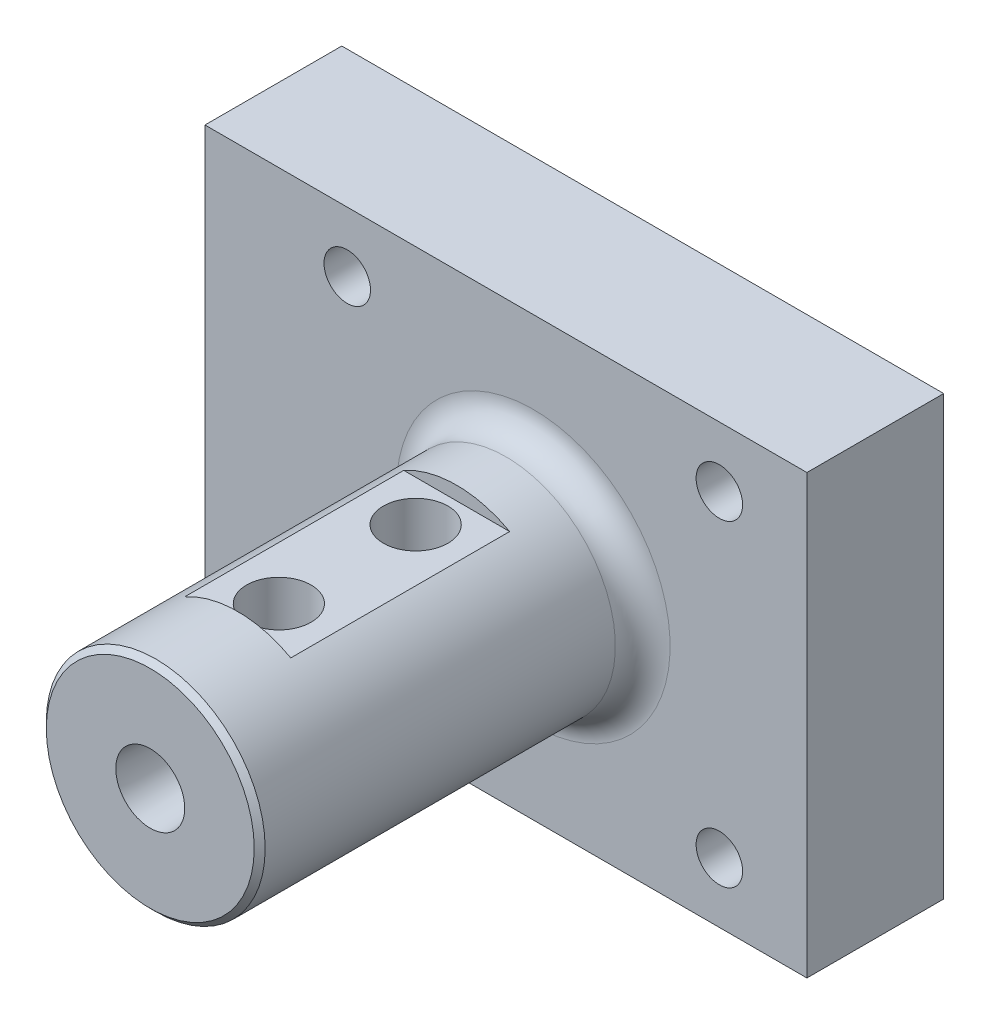
SolidWorks part; units mm, degrees
material "T2"
ref_plane "前视基准面" through (0, 0, 0) normal (0, 0, 1) x (1, 0, 0)
ref_plane "上视基准面" through (0, 0, 0) normal (0, 1, 0) x (1, 0, 0)
ref_plane "右视基准面" through (0, 0, 0) normal (1, 0, 0) x (0, 0, -1)
sketch "草图13" plane through (0, 0, 0) normal (0, 0, 1) x (1, 0, 0)
  line L1 (-50, -40) -> (50, -40)
  line L2 (-50, -40) -> (-50, 40)
  line L3 (-50, 40) -> (50, 40)
  line L4 (50, -40) -> (50, 40)
  line L5 (0, 40) -> (0, -40) construction
  line L6 (-50, 0) -> (50, 0) construction
  point P0 (0, 0)
  dimension "D1" = 100
  dimension "D2" = 80
extrude "凸台-拉伸3" add sketch "草图13" along normal blind 25
sketch "草图14" plane through (0, 0, 25) normal (0, 0, 1) x (1, 0, 0)
  line L1 (-34, -29) -> (34, -29) construction
  line L2 (-34, -29) -> (-34, 29) construction
  line L3 (-34, 29) -> (34, 29) construction
  line L4 (34, -29) -> (34, 29) construction
  line L5 (0, 29) -> (0, -29) construction
  line L6 (-34, 0) -> (34, 0) construction
  circle A0 centre (-34, 29) radius 0.5
  circle A1 centre (34, 29) radius 0.5
  circle A2 centre (34, -29) radius 0.5
  circle A3 centre (-34, -29) radius 0.5
  point P0 (0, 0)
  dimension "D3" = 1
  dimension "D1" = 68
  dimension "D2" = 58
extrude "切除-拉伸4" cut sketch "草图14" against normal blind 18
sketch "草图15" plane through (0, 0, 25) normal (0, 0, 1) x (1, 0, 0)
  circle A0 centre (0, 0) radius 20
  dimension "D1" = 40
extrude "凸台-拉伸4" add sketch "草图15" along normal blind 70
hole_wizard "Ø10.0 (10) 直径孔1" positions "草图16" profile "草图17" hole size "Ø10.0" standard "GB"
sketch "草图16" plane through (0, 0, 95) normal (0, 0, 1) x (1, 0, 0)
  point P5 (0, 0)
sketch "草图17" plane through (0, 0, 95) normal (1, 0, 0) x (0, -1, 0)
  line L0 (0, 0) -> (0, 28.0043)
  line L1 (0, 28.0043) -> (5, 25)
  line L2 (5, 25) -> (5, 0)
  line L5 (5, 0) -> (0, 0)
  line L10 (0, 28.0043) -> (-5, 25) construction
  line L11 (0, -6.35) -> (0, 107.95) construction
  dimension "孔直径" = 10
  dimension "孔深度" = 25
  dimension "导头角度" = 118
sketch "草图19" plane through (0, 0, 0) normal (0, 1, 0) x (1, 0, 0)
  line L0 (0, -95) -> (0, 0) construction
  line L1 (-20, -95) -> (20, -95) construction
  line L2 (0, -95) -> (-0.5, -95) construction
  line L3 (-0.5, -95) -> (0, -85) construction
  line L4 (0, -95) -> (-0.5, -95)
  line L5 (-6.3, -95) -> (-5.65, -82)
  line L6 (-5.65, -82) -> (-5, -82)
  line L8 (-5, -82) -> (-5, -95)
  line L10 (0, -95) -> (-0.5, -95)
  line L11 (-5, -70) -> (-5, -95) construction
  line L12 (-5, -95) -> (-6.3, -95)
  dimension "D1" = 0.5
  dimension "D2" = 10
  dimension "D3" = 12.6
  dimension "D4" = 13
revolve "切除-旋转10" cut sketch "草图19" angle 360 about L0
ref_plane "基准面3" through (0, 0, 79) normal (0, 0, 1) x (1, 0, 0)
sketch "草图21" plane through (0, 0, 79) normal (0, 0, 1) x (1, 0, 0)
  line L1 (-27.2886, -17.5) -> (27.2886, -17.5)
  line L2 (-27.2886, -17.5) -> (-27.2886, 17.5)
  line L3 (-27.2886, 17.5) -> (27.2886, 17.5)
  line L4 (27.2886, -17.5) -> (27.2886, 17.5)
  line L5 (0, 17.5) -> (0, -17.5) construction
  line L6 (-27.2886, 0) -> (27.2886, 0) construction
  point P0 (0, 0)
  dimension "D1" = 35
extrude "切除-拉伸5" cut sketch "草图21" against normal blind 40 flip side to cut
hole_wizard "G1/4 螺纹孔1" positions "草图22" profile "草图23" tap size "G1/4" standard "GB"
sketch "草图22" plane through (0, 17.5, 0) normal (0, 1, 0) x (1, 0, 0)
  line L0 (0, 0) -> (0, -95) construction
  line L1 (-20, -95) -> (20, -95) construction
  line L2 (-9.6825, -59) -> (9.6825, -59) construction
  line L3 (-9.6825, -39) -> (-9.6825, -79) construction
  line L4 (9.6825, -79) -> (9.6825, -39) construction
  point P13 (0, -46.5)
  point P15 (0, -71.5)
  dimension "D1" = 25
sketch "草图23" plane through (0, 17.5, 71.5) normal (1, 0, 0) x (0, 0, 1)
  line L0 (0, 0) -> (0, 28.5451)
  line L1 (0, 28.5451) -> (5.9, 25)
  line L2 (5.9, 25) -> (5.9, 0)
  line L5 (5.9, 0) -> (0, 0)
  line L10 (0, 28.5451) -> (-5.9, 25) construction
  line L11 (0, -6.35) -> (0, 107.95) construction
  dimension "螺纹孔钻头直径" = 11.8
  dimension "螺纹孔钻头深度" = 25
  dimension "导头角度" = 118
cosmetic thread "孔螺蚊线5" parameters "D1"=20, "D2"=13.157
cosmetic thread "孔螺蚊线6" parameters "D1"=20, "D2"=13.157
chamfer "倒角1" distance 1 angle 45 1 edges at (20, 0, 95)
hole_wizard "M10 螺纹孔1" positions "草图24" profile "草图25" tap size "M10" standard "GB"
sketch "草图24" plane through (0, 0, 25) normal (0, 0, 1) x (1, 0, 0)
  point P4 (-34, 29)
  point P7 (34, 29)
  point P10 (34, -29)
  point P13 (-34, -29)
sketch "草图25" plane through (-34, 29, 25) normal (1, 0, 0) x (0, -1, 0)
  line L0 (0, 0) -> (0, 30.0537)
  line L1 (0, 30.0537) -> (4.25, 27.5)
  line L2 (4.25, 27.5) -> (4.25, 0)
  line L5 (4.25, 0) -> (0, 0)
  line L10 (0, 30.0537) -> (-4.25, 27.5) construction
  line L11 (0, -6.35) -> (0, 107.95) construction
  dimension "螺纹孔钻头直径" = 8.5
  dimension "螺纹孔钻头深度" = 27.5
  dimension "导头角度" = 118
cosmetic thread "孔螺蚊线7" parameters "D1"=18, "D2"=10
cosmetic thread "孔螺蚊线8" parameters "D1"=18, "D2"=10
cosmetic thread "孔螺蚊线9" parameters "D1"=18, "D2"=10
cosmetic thread "孔螺蚊线10" parameters "D1"=18, "D2"=10
fillet "圆角1" radius 5 1 edges at (-20, 0, 25)
ref_plane "基准面4" through (0, 0, 69) normal (0, 0, 1) x (1, 0, 0)
hole_wizard "M6 螺纹孔1" positions "草图26" profile "草图27" tap size "M6" standard "GB"
sketch "草图26" plane through (0, 0, 69) normal (0, 0, 1) x (1, 0, 0)
  point P0 (0, 0)
sketch "草图27" plane through (0, 0, 69) normal (1, 0, 0) x (0, -1, 0)
  line L0 (0, 0) -> (0, 36.5022)
  line L1 (0, 36.5022) -> (2.5, 35)
  line L2 (2.5, 35) -> (2.5, 0)
  line L5 (2.5, 0) -> (0, 0)
  line L10 (0, 36.5022) -> (-2.5, 35) construction
  line L11 (0, -6.35) -> (0, 107.95) construction
  dimension "螺纹孔钻头直径" = 5
  dimension "螺纹孔钻头深度" = 35
  dimension "导头角度" = 118
cosmetic thread "孔螺蚊线11" parameters "D1"=30, "D2"=6
sketch "草图29" plane through (-50, 0, 0) normal (-1, 0, 0) x (0, 0, 1)
  line L4 (0, 40) -> (0, -40)
  line L5 (0, -40) -> (25, -40)
  line L6 (25, -40) -> (25, 40)
  line L7 (25, 40) -> (0, 40)
  line L8 (0, 40) -> (0, -40)
  line L9 (0, -40) -> (25, -40)
  line L10 (25, -40) -> (25, 40)
  line L11 (25, 40) -> (0, 40)
  dimension "D1" = 0
extrude "凸台-拉伸5" add sketch "草图29" along normal blind 10
hole_wizard "M10 螺纹孔2" positions "草图30" profile "草图31" tap size "M10" standard "GB"
sketch "草图30" plane through (-60, 0, 0) normal (-1, 0, 0) x (0, 0, 1)
  line L0 (0, 0) -> (25, 0) construction
  line L1 (25, -40) -> (25, 40) construction
  line L2 (12.5, 40) -> (12.5, -40) construction
  line L3 (25, 40) -> (0, 40) construction
  line L4 (0, -40) -> (25, -40) construction
  point P17 (12.5, 18)
  point P19 (12.5, -18)
  point P22 (0, 0)
  dimension "D1" = 36
sketch "草图31" plane through (-60, -18, 12.5) normal (0, 1, 0) x (0, 0, 1)
  line L0 (0, 0) -> (0, 30.0537)
  line L1 (0, 30.0537) -> (4.25, 27.5)
  line L2 (4.25, 27.5) -> (4.25, 0)
  line L5 (4.25, 0) -> (0, 0)
  line L10 (0, 30.0537) -> (-4.25, 27.5) construction
  line L11 (0, -6.35) -> (0, 107.95) construction
  dimension "螺纹孔钻头直径" = 8.5
  dimension "螺纹孔钻头深度" = 27.5
  dimension "导头角度" = 118
cosmetic thread "孔螺蚊线12" parameters "D1"=20, "D2"=10
cosmetic thread "孔螺蚊线13" parameters "D1"=20, "D2"=10
